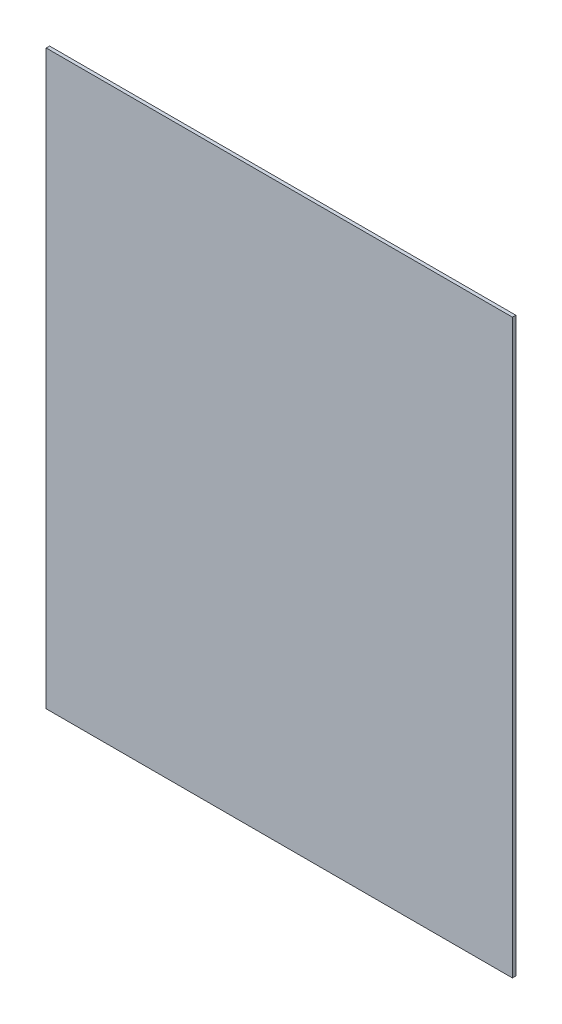
from build123d import *

# Parameters (mm, degrees)
SKETCH_1_W      = 686
SKETCH_1_H      = 842
EXTRUDE_1_DEPTH = 5


with BuildPart() as part:
    # 草图1 → 凸台-拉伸1 (new body)
    with BuildSketch(Plane.XY):
        Rectangle(SKETCH_1_W, SKETCH_1_H)
    extrude(amount=EXTRUDE_1_DEPTH)


solid = part.part
